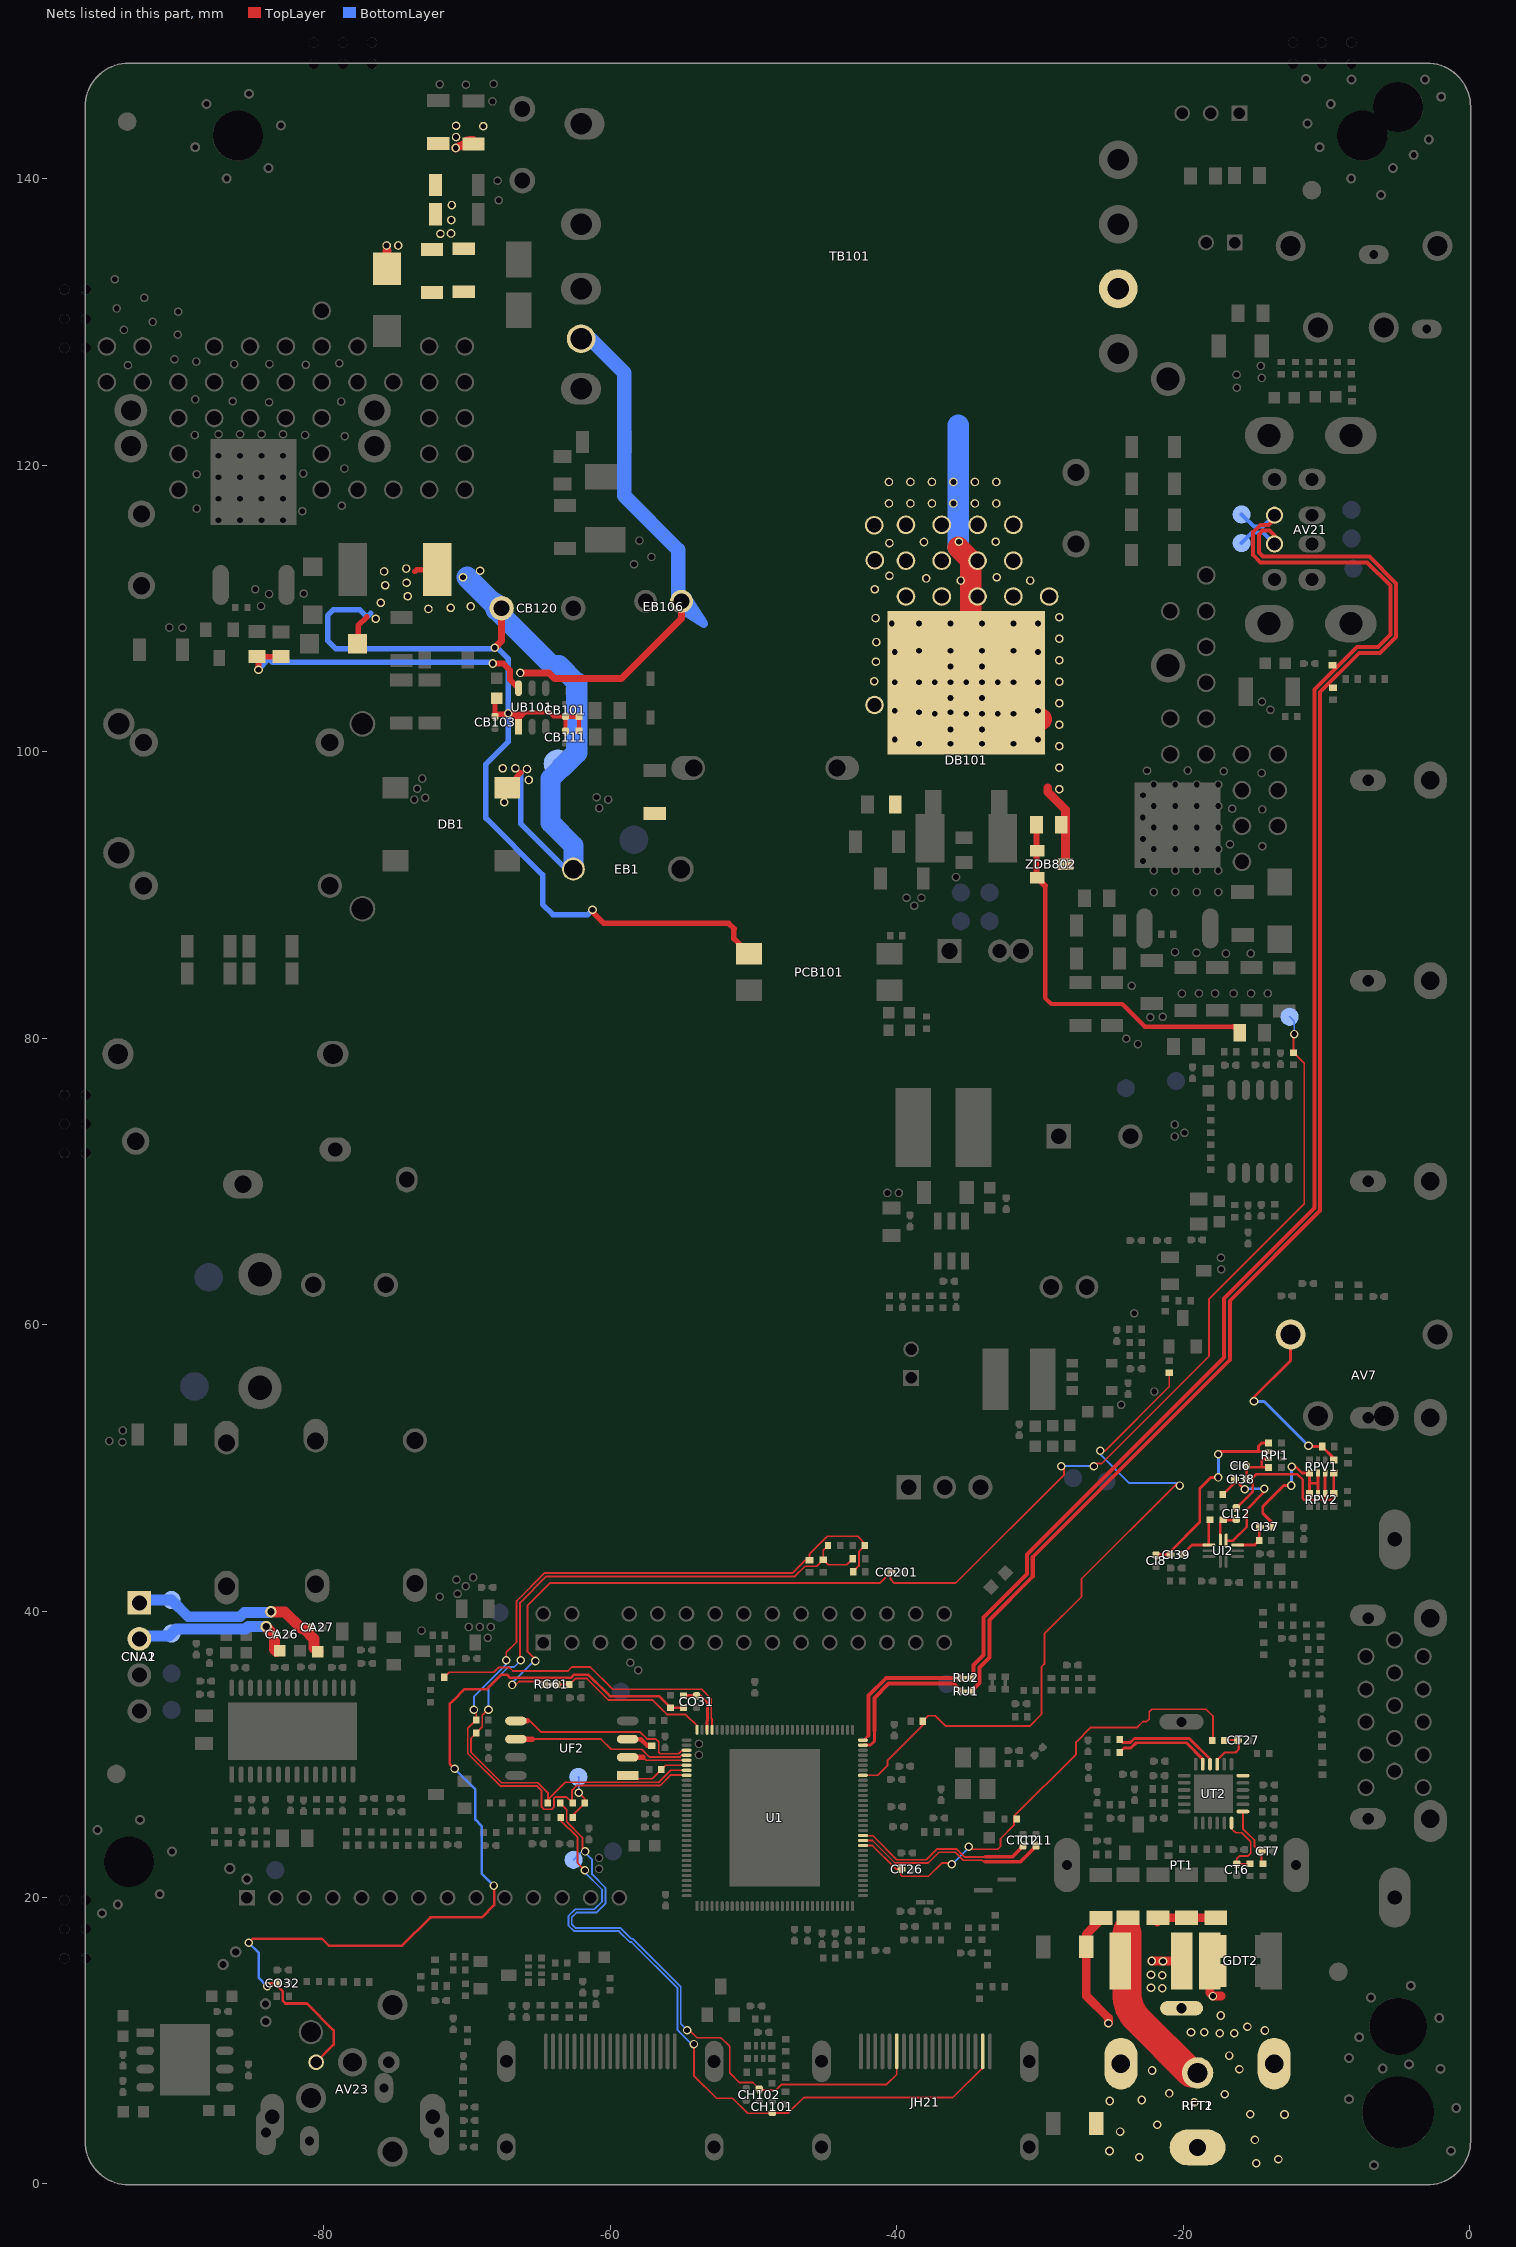
[diagram p0: the nets of this part, all layers, seen from the top]
# Altium PCB MISC86372.PcbDoc (part 13 of 16)
Units mm, origin at the board's own origin, x right, y up, seen from the top; angles counter-clockwise.
Board outline 96.73 x 148.13 mm, 2 copper layers (TopLayer, BottomLayer), stack 1.571 mm thick; 578 components, 318 nets, 2702 pads, 836 vias.

## Via types
v1: diameter 0.6, hole 0.4, TopLayer to BottomLayer, tented both sides, 816 vias
v2: diameter 0.7, hole 0.5, TopLayer to BottomLayer, tented both sides, 15 vias
v3: diameter 0.8, hole 0.5, TopLayer to BottomLayer, tented both sides, 5 vias

## Nets (pads, with @x,y where several pads share a name; then routed paths per layer and width w, separated by ;. In a path a pad name is that pad's centre, name@x,y a point inside that pad or via, vN(x,y) a via of type N, cw(c..) or ccw(c..) an arc to the next point about the centre after c; other vN are vias at no path point) (continued)
NetRB106_1: RB106.1 RB107.1 UB101.6 | length 23.3
  TopLayer w0.4: v1(-84.557,105.715) -84.557,106.627 -84.554,106.624 RB107.1@-82.982,106.624 ; -83.871,106.627 RB107.1@-82.906,106.627 ; v1(-68.199,106.147) -67.469,106.147 -66.996,105.674 -66.996,105.017 UB101.6@-66.406,104.427
  BottomLayer w0.4: v1(-84.557,105.715) -84.607,105.715 -83.829,106.493 -83.565,106.229 -68.281,106.229 v1(-68.199,106.147)
NetRB834_2: RB834.2 RB835.2 ZDB802.1 ZDB802.3 | length 26.9
  TopLayer w0.3: -29.642,90.627 -29.642,82.804 -29.211,82.373 -24.258,82.373 -22.682,80.797 RB834.2@-16.487,80.797
  TopLayer w0.4: RB835.2@-30.251,94.894 -30.251,91.237 ZDB802.3@-30.201,91.186 -29.642,90.627 ; RB834.2@-16.487,80.797 RB834.2@-16.055,80.366
NetRF23_1: RF23.1 UF2.3 | length 1.9
  TopLayer w0.305: UF2.3@-58.787,31.055 -57.869,31.055 -57.419,30.604 RF23.1@-57.099,30.604
NetRH102_2: RH102.2 RH105.1 RXD.1 | length 3.5
  TopLayer w0.127: RH102.2@-62.669,25.578 -62.669,25.705 RH105.1@-61.78,26.594 -61.78,26.88 v1(-62.205,27.305) v1@-62.255,27.254
  BottomLayer w0.127: RXD.1@-62.23,28.423 -62.205,28.397 v1(-62.205,27.305)
PANEL_EN_OUT_IC: RM11.1 U1.93 | length 22.3
  TopLayer w0.127: RM11.1@-71.603,35.377 -71.248,35.731 -68.136,35.731 -67.8,36.068 -67.048,36.068 -66.794,35.814 -62.956,35.814 -62.677,36.093 -61.392,36.093 -59.833,34.535 -56.159,34.535 -53.627,34.535 -52.952,33.86 -52.952,32.505 -52.885,32.438 -52.888,32.434 U1.93@-52.888,31.707 U1.93@-52.888,31.656
PC_L&AV_L: CI37.2@-13.85,45.868 CI37.2@-14.025,45.868 RPV1.6 RPV1.8 RPV2.2 RPV2.4 | length 10.4
  TopLayer w0.203: CI37.2@-13.85,45.868 -13.85,46.234 -14.448,46.832 -14.448,47.3 -12.983,48.765 v1(-12.453,48.765) ; v1(-12.421,50.063) -12.135,50.063 -11.703,49.632 RPV1.8@-11.192,49.632 -11.192,48.92 ; RPV2.2@-11.192,48.209 -11.192,48.692 -11.192,48.92 ; RPV2.4@-10.592,48.209 -10.592,48.946 ; RPV1.6@-10.592,49.632 -10.592,48.946 ; -11.192,48.92 -10.617,48.92 -10.592,48.946
  BottomLayer w0.203: v1(-12.453,48.765) v1@-12.453,50.031
PC_LIN_SW: CI37.1 RI37.1 UI2.10 | length 2.6
  TopLayer w0.178: UI2.10@-16.206,44.608 -15.02,44.608 RI37.1@-14.7,44.929 CI37.1@-14.7,45.868
PC_R: AV7.3 DV8.K RPV1.1 | length 13.7
  TopLayer w0.203: v1(-15.062,54.635) -15.062,54.933 -12.5,57.495 AV7.3@-12.5,59.3 AV7.3@-12.776,59.024 ; v1@-11.201,51.486 DV8.K@-10.306,51.486 -9.492,50.672 RPV1.1@-9.492,50.532
  BottomLayer w0.203: v1(-15.062,54.635) -14.351,54.635 v1@-11.328,51.613 ; AV7.3@-12.802,58.998 AV7.3@-12.5,59.3
  other v1: -11.252,51.537
PC_R&AV_R: CI12.2@-16.298,47.23 CI12.2@-16.298,47.055 RPV1.2 RPV1.4 RPV2.6 RPV2.8 | length 13.8
  TopLayer w0.178: CI12.2@-16.298,47.23 -16.245,47.23 -15.161,48.313 -15.161,49.276 -14.877,49.56 -12.044,49.56 -11.658,49.174 -11.658,47.87 -11.547,47.759 -10.178,47.759 ; RPV2.6@-10.092,48.209 -10.084,48.201 -10.084,47.854 -10.178,47.759 ; RPV1.4@-10.092,49.632 RPV1.4@-10.092,49.801 ; RPV2.8@-9.492,48.209 -9.492,47.836 -9.569,47.759 -10.178,47.759
  TopLayer w0.203: RPV2.6@-10.092,48.209 RPV1.4@-10.092,49.632 ; RPV2.8@-9.492,48.209 RPV1.2@-9.492,49.632
PC_RIN_SW: CI12.1 RI38.1 UI2.2 | length 2.3
  TopLayer w0.178: UI2.2@-17.406,44.958 -17.406,46.186 RI38.1@-17.213,46.38 ; -16.838,46.352 -16.836,46.354
  TopLayer w0.203: RI38.1@-17.085,46.354 -16.836,46.354 ; -16.838,46.352 -16.326,46.352 CI12.1@-16.298,46.38
POWER_EN_OUT_IC: RM1.1 RM2.1 U1.57 | length 49.4
  TopLayer w0.127: U1.57@-42.362,28.531 -41.327,28.531 -40.653,29.204 -40.653,29.541 RM1.1@-38.101,32.093 ; RM1.1@-38.183,32.309 -37.803,32.689 -37.309,32.689 -36.59,31.97 -30.728,31.97 -29.893,32.804 -29.893,36.108 -29.693,36.309 -29.693,38.405 -27.102,40.996 -27.102,42.24 v1@-20.418,48.924 ; v1(-25.794,51.194) -25.46,51.194 -20.98,55.673 RM2.1@-20.98,56.623
  BottomLayer w0.127: v1(-25.794,51.194) -25.794,50.947 -23.78,48.933 -20.426,48.933 v1(-20.25,48.757)
PWM1: RF13.1 RG61.1 U1.96 | length 11.6
  TopLayer w0.127: RG61.1@-63.71,34.87 RF13.1@-62.858,34.87 -62.443,35.285 -61.625,35.285 -60.122,33.782 -57.039,33.782 -56.413,33.157 -56.032,32.775 -55.711,32.775 -55.702,32.766 -54.725,32.766 -53.938,31.979 U1.96@-53.938,31.707 U1.96@-53.938,31.656
PWM_REF: CG201.1 PWM_REF.1 RB813.1 RG61.2 RG61.3 | length 92.7
  TopLayer w0.127: v1@-66.754,34.693 -66.37,35.077 -64.767,35.077 RG61.2@-64.56,34.87 ; -65.786,37.795 -65.786,38.278 ; v1(-65.227,36.508) -65.227,36.627 -65.786,37.186 -65.786,38.278 ; v1@-28.321,49.911 -28.321,49.527 -35.897,41.951 -40.173,41.951 -40.43,42.208 CG201.1@-40.43,42.723 -41.201,41.951 -64.215,41.951 -65.786,40.38 -65.786,38.278 ; v1@-26.054,50.298 -25.698,50.298 -18.194,57.802 -18.194,61.79 -11.557,68.427 -11.557,78.251 RB813.1@-12.294,78.987 -12.294,80.233 v1(-12.248,80.278) v1@-12.248,80.309
  BottomLayer w0.127: v1(-66.837,34.841) -66.837,34.992 -66.345,35.484 ; v1@-66.754,35.075 -66.345,35.484 ; v1@-65.275,36.555 -66.345,35.484 ; v1(-28.524,50.114) v1(-26.238,50.114) ; PWM_REF.1@-12.573,81.483 -12.248,81.159 v1(-12.248,80.278)
RF_INPUT: CT13.1 GDT1.1 RFT1.1 RFT2.1 | length 12.2
  TopLayer w1.905: GDT1.1@-23.933,17.522 -23.933,17.767
  TopLayer w2.032: GDT1.1@-23.925,17.514 -23.925,13.267 ccw(c-21.385,13.267) -23.181,11.471 -19.461,7.75 RFT1.1@-19,7.75
RFGND: CT41.2 CT42.2 CT43.2 CT44.2 CT45.2 CT46.2 CT47.2 CT48.2 GDT1.2 GDT2.1@-17.501,14.554 GDT2.1@-17.502,16.586 GDT2.1@-18.152,15.57 PT1.1 RFT1.2 RFT1.3 RFT1.4 RFT2.2 RFT2.3 RFT2.4 | length 18
  TopLayer w0.61: CT41.2@-25.754,18.566 -25.754,18.446 -26.77,17.43 CT47.2@-26.77,16.561 -26.77,13.13 -25.222,11.582 v1(-25.222,11.227) ; v1(-22.2,15.57) GDT1.2@-20.1,15.57 ; CT42.2@-21.817,18.289 -21.817,18.591 CT44.2@-17.753,18.591 ; GDT2.1@-18.152,15.57 -18.152,13.343 v1(-17.927,13.118) -17.342,13.118
  other v1: -14.901,1.448 -13.356,1.727 -23.067,1.86 -25.146,2.3 -14.994,3.076 -24.409,3.658 -21.819,4.14 -12.929,4.851 -15.316,4.877 -19.228,5.69 -25.132,5.791 -22.9,5.865 -17.094,6.274 -20.98,6.325 -22.173,7.924 -16.078,8.001 -16.789,8.966 -17.45,10.516 -16.434,10.516 -19.456,10.59 -18.542,10.592 -14.3,10.718 -15.519,10.973 -17.374,11.76 -21.463,13.665 -22.25,13.691 -21.463,14.58 -22.25,14.605 -21.412,15.545
ROUT+: BA4.2 CA27.1 CNA1.1 CNA2.1 pad.VIA5@-83.693,39.954 ROUT+.1 | length 14.6
  TopLayer w0.762: pad.VIA5@-83.693,39.929 -82.724,39.929 -81.563,38.767 -81.4,38.767 -80.683,38.051 -80.683,37.432 BA4.2@-80.412,37.16
  BottomLayer w0.762: CNA1.1@-92.877,40.773 -90.634,40.773 ROUT+.1@-90.627,40.767 -89.462,39.601 -85.855,39.601 -85.553,39.903 pad.VIA5@-83.693,39.903
ROUT-: BA3.2 CA26.2@-83.177,38.372 CA26.2@-83.352,38.372 CNA1.2 CNA2.2 pad.VIA5@-84.023,38.913 ROUT-.1 | length 10.9
  TopLayer w0.254: -83.687,37.668 -83.687,38.179
  TopLayer w0.762: pad.VIA5@-84.023,38.913 -84.023,38.875 -83.687,38.538 ; -83.433,37.922 -83.433,37.322 BA3.2@-83.298,37.188
  BottomLayer w0.762: CNA1.2@-92.877,38.253 -90.804,38.253 ROUT-.1@-90.627,38.43 -90.32,38.738 -85.468,38.738 -85.293,38.913 pad.VIA5@-84.023,38.913
RXD: CH101.2@-48.692,4.96 CH101.2@-48.692,5.135 JH21.2 RH102.1 | length 50
  TopLayer w0.127: RH102.1@-63.519,25.578 -63.519,25.441 -62.281,24.204 -62.281,22.403 v1(-61.773,21.895) ; v1(-54.161,9.765) -54.161,7.57 -52.583,5.991 -51.465,5.991 -50.413,4.938 -49.298,4.938 ; -49.294,4.942 -48.819,4.942 -48.819,4.96 -47.566,4.96 -46.488,6.037 -36.09,6.037 -34,8.127 JH21.2@-34,9.258
  BottomLayer w0.127: v1@-61.773,21.753 -60.579,20.559 -60.579,19.714 -61.116,19.177 -62.452,19.177 -62.916,18.713 -62.916,18.041 -62.528,17.653 -59.398,17.653 -58.636,16.891 -58.522,16.891 -55.304,13.673 -55.304,10.743 v1@-54.326,9.765
SC_AU_LIN_C: CI6.2@-15.582,50.126 CI6.2@-15.757,50.126 CI38.2@-15.577,49.2 CI38.2@-15.752,49.2 RPI1.2 RPI1.4 | length 3.5
  TopLayer w0.178: -15.582,49.842 CI6.2@-15.582,50.126 ; CI38.2@-15.577,49.2 -15.582,49.205 CI6.2@-15.582,50.126 ; -14.503,50.063 -14.503,50.521 -14.398,50.626 -14.308,50.626 ; RPI1.2@-14.039,50.026 -15.482,50.026 CI6.2@-15.582,50.126
SC_AU_LIN_SW: CI38.1 RI39.1 UI2.1 | length 8.9
  TopLayer w0.178: RI39.1@-17.228,48.148 RI39.1@-17.228,48.133 -16.427,48.934 ; UI2.1@-17.006,44.908 -16.526,44.908 -15.553,45.882 -15.553,47.096 -14.351,48.297 v1(-14.351,48.539) ; -16.427,48.913 CI38.1@-16.427,49.2 -15.724,48.497 v1(-15.711,48.497) ; CI38.1@-16.252,49.124 CI38.1@-16.252,49.2
  BottomLayer w0.178: v1(-15.711,48.497) -15.669,48.539 v1(-14.351,48.539)
SC_AU_RIN_C: CI8.2@-21.895,43.76 CI8.2@-21.895,43.935 CI39.2@-20.752,43.94 CI39.2@-20.927,43.94 RPI1.6 RPI1.8 | length 14.3
  TopLayer w0.203: CI8.2@-21.895,43.935 CI39.2@-20.931,43.935 ; CI39.2@-20.927,44.124 -18.847,46.204 -18.847,48.561 -18.081,49.327 v1(-17.552,49.327) ; v1(-17.552,50.952) -17.378,51.126 -16.951,51.126 ; -16.971,51.126 -16.951,51.126 ; RPI1.6@-14.039,51.126 -14.732,51.126 ; RPI1.8@-14.039,51.726 -14.523,51.726 -14.732,51.517 -14.732,51.126 ; -16.951,51.126 -14.732,51.126
  BottomLayer w0.203: v1@-17.544,49.327 v1@-17.544,50.952
SC_AU_RIN_SW: CI39.1 RI40.1 UI2.3 | length 4
  TopLayer w0.178: -19.379,44.608 UI2.3@-18.206,44.608 -18.206,46.301 RI40.1@-18.127,46.38
  TopLayer w0.203: CI39.1@-20.098,43.889 -19.379,44.608
SGND: CB101.2@-63.129,102.62 CB101.2@-63.129,102.445 CB102.2 CB103.2@-68.047,102.282 CB103.2@-68.047,102.457 CB111.1 CB120.1 DB1.4 DB110.K EB1.2@-62.576,91.796 EB106.2 pad.VIA5@-65.684,98.019 pad.VIA5@-65.811,98.781 pad.VIA5@-66.624,98.831 pad.VIA5@-67.412,96.469 pad.VIA5@-67.513,98.831 pad.VIA5@-69.088,112.624 pad.VIA5@-69.748,110.134 pad.VIA5@-70.282,112.166 pad.VIA5@-71.145,110.033 pad.VIA5@-72.695,109.957 pad.VIA5@-74.143,110.846 pad.VIA5@-74.219,111.785 pad.VIA5@-74.244,112.776 pad.VIA5@-75.717,111.608 pad.VIA5@-75.794,112.573 pad.VIA5@-76.022,110.388 pad.VIA5@-76.378,109.271 PCB101.3 RB103.1 RB104.1 RB130.1 RB148.1 TB101.5 TP-TDT.2 UB101.1 | length 143.7
  TopLayer w0.3: UB101.1@-66.406,102.245 -65.927,102.724 -64.237,102.724 -63.957,102.445 CB101.2@-63.129,102.445 ; -63.129,101.847 CB111.1@-63.129,101.441 CB101.2@-63.129,102.445 ; RB104.1@-62.189,101.441 RB103.1@-62.189,102.42 -63.103,102.42 CB101.2@-63.129,102.445
  TopLayer w0.381: DB110.K@-77.597,107.366 -77.597,108.788 -76.987,109.398 ; -73.635,112.573 -73.508,112.7 RB148.1@-72.082,112.7 ; CB103.2@-68.047,102.562 CB102.2@-68.047,103.815 ; CB103.2@-68.021,102.591 -66.751,102.591 ; DB1.4@-66.878,97.892 -66.243,98.527 ; UB101.1@-66.406,102.245 -66.751,102.591 ; -66.142,102.591 -66.751,102.591 ; v1(-61.239,88.951) -61.239,88.794 -60.452,88.007 -51.731,88.007 -51.358,87.634 -51.365,87.627 -51.365,86.944 -49.957,85.536 PCB101.3@-49.957,85.522
  TopLayer w0.5: v1(-68.072,107.239) -67.586,107.725 CB120.1@-67.586,110.007 ; v1(-66.29,105.49) -64.274,105.49 -63.89,105.105 -59.207,105.105 -55.031,109.282 EB106.2@-55.031,110.49
  BottomLayer w0.381: -76.721,109.664 -76.987,109.398 -77.495,109.906 -79.324,109.906 -79.731,109.499 -79.731,107.74 -79.177,107.186 v1@-68.072,107.186 ; v1@-67.835,107.186 -67.132,106.483 v1(-67.132,102.667) -67.132,100.677 -68.682,99.128 -68.682,95.352 -64.719,91.389 -64.719,89.332 -64.008,88.621 -61.57,88.621 v1(-61.239,88.951) ; -66.243,98.527 -66.243,94.945 -63.094,91.796 EB1.2@-62.576,91.796
  BottomLayer w1: TB101.5@-62.038,128.819 -61.408,128.819 -59.03,126.441 -59.03,117.856 -55.265,114.091 EB106.2@-55.265,110.236
  BottomLayer w1.4: CB120.1@-67.829,109.764 -64.096,106.032 -63.573,106.032 -62.357,104.816 ; TP-TDT.2@-63.076,99.205 -64.16,98.12 -64.16,95.021 -62.576,93.437 EB1.2@-62.576,91.796
  BottomLayer w1.5: pad.VIA5@-69.999,112.166 CB120.1@-67.958,110.126 ; CB120.1@-67.958,109.894 CB120.1@-67.958,110.126 ; CB120.1@-67.586,109.753 CB120.1@-67.958,110.126 ; TP-TDT.2@-63.39,98.89 -62.357,99.924 -62.357,104.816
SNB-D: DB106.K pad.VIA5@-68.859,143.662 pad.VIA5@-70.79,142.138 pad.VIA5@-70.764,142.9 pad.VIA5@-70.764,143.688 pad.VIA5@-74.803,135.331 pad.VIA5@-75.616,135.331 RB117.1 RB118.1 RB150.1 RB151.1 | length 3.3
  TopLayer w0.6: DB106.K@-75.59,133.706 -75.59,134.976 ; pad.VIA5@-70.79,142.138 RB117.1@-69.897,142.54 ; RB117.1@-69.774,142.416 RB117.1@-69.897,142.54 ; RB117.1@-69.897,142.54 -69.672,142.641 -69.629,142.66 -69.586,142.68 -69.799,142.667 -70.004,142.646 RB117.1@-69.897,142.54
SNB-RM: pad.VIA5@-71.12,136.169 pad.VIA5@-71.065,138.151 pad.VIA5@-71.095,137.109 pad.VIA5@-71.857,136.144 RB150.2 RB151.2 RB152.1 RB153.1
SPDIF_OUT: AV23.1 CO32.2@-83.28,14.021 CO32.2@-83.105,14.021 RO21.2 RO22.2 | length 65.4
  TopLayer w0.178: v1(-85.242,16.84) -84.963,17.12 -80.137,17.12 -79.654,16.637 -74.534,16.637 -72.553,18.618 -68.971,18.618 -68.116,19.473 v1@-68.116,20.805 ; v1(-83.952,13.797) -83.728,14.021 CO32.2@-83.28,14.021 ; CO32.2@-83.28,13.851 -82.855,13.426 -82.855,12.776 -82.677,12.598 -81.178,12.598 -79.308,10.728 -79.308,9.732 AV23.1@-80.54,8.5 ; v1(-70.872,28.989) -71.144,29.262 -71.222,29.339 -71.222,33.506 -70.995,33.733 -70.184,34.544 -68.605,34.544 -67.589,35.56 -67.222,35.56 -66.993,35.331 -62.756,35.331 -62.528,35.56 -61.541,35.56 -61.026,35.046 ; -61.287,35.306 -60.033,34.052 -56.6,34.052 RO22.2@-55.804,33.255 RO22.2@-55.702,33.255 ; RO22.2@-55.753,33.306 RO22.2@-55.702,33.255 ; RO22.2@-55.695,33.249 RO22.2@-55.702,33.255 ; RO21.2@-54.88,33.249 -54.886,33.255 RO22.2@-55.702,33.255
  BottomLayer w0.178: v1(-85.242,16.84) -84.557,16.154 -84.557,14.401 v1(-83.952,13.797) ; v1(-70.872,28.989) -69.425,27.542 -69.425,25.432 -68.982,24.989 -68.982,21.671 v1(-68.144,20.833)
SPDIF_OUT_IC: CO31.2@-53.975,33.931 CO31.2@-53.975,34.106 RO21.1 U1.94 | length 3.8
  TopLayer w0.203: RO21.1@-54.845,34.163 -54.788,34.106 CO31.2@-53.975,34.106 ; CO31.2@-53.95,34.106 CO31.2@-53.975,34.106 ; U1.94@-53.238,31.656 U1.94@-53.238,31.707 -53.238,32.334 -53.219,32.354 -53.219,33.615 -53.709,34.106 CO31.2@-53.975,34.106
SPI_CLK: U1.100 UF2.6 | length 12.6
  TopLayer w0.127: -65.441,31.055 -60.646,31.055 -59.944,30.353 -57.809,30.353 -57.265,29.809 -55.138,29.809 -55.016,29.931 U1.100@-54.663,29.931
  TopLayer w0.381: UF2.6@-66.707,31.055 -65.441,31.055
SPI_CSN: RF3.1 U1.102 UF2.1 | length 4.6
  TopLayer w0.127: UF2.1@-58.787,28.515 -58.559,28.286 -57.085,28.286 RF3.1@-56.44,28.931 -56.14,29.231 U1.102@-54.664,29.231
SPI_DI: U1.99 UF2.5 | length 13.4
  TopLayer w0.127: -65.799,32.325 -65.619,32.325 -64.857,31.563 -57.928,31.563 -57.429,31.064 -56.82,31.064 -56.617,30.861 -56.617,30.15 -56.505,30.038 -55.232,30.038 -54.99,30.281 U1.99@-54.613,30.281
  TopLayer w0.381: UF2.5@-66.587,32.325 -65.799,32.325
SPI_DO: U1.101 UF2.2 | length 4.2
  TopLayer w0.127: -57.744,29.785 -57.699,29.785 -57.495,29.581 U1.101@-54.664,29.581
  TopLayer w0.381: UF2.2@-58.787,29.785 -57.744,29.785
SYN: CB117.1 DB101.2 pad.VIA5@-28.651,97.378 pad.VIA5@-28.651,98.878 pad.VIA5@-28.651,100.378 pad.VIA5@-28.651,101.878 pad.VIA5@-28.651,103.378 pad.VIA5@-28.651,104.878 pad.VIA5@-28.651,106.378 pad.VIA5@-28.651,107.878 pad.VIA5@-28.651,109.378 pad.VIA5@-29.359,110.827 pad.VIA5@-30.683,111.938 pad.VIA5@-31.859,110.827 pad.VIA5@-31.859,113.327 pad.VIA5@-31.859,115.827 pad.VIA5@-33.02,112.166 pad.VIA5@-33.045,117.321 pad.VIA5@-33.045,118.821 pad.VIA5@-33.096,114.656 pad.VIA5@-34.359,110.827 pad.VIA5@-34.359,113.327 pad.VIA5@-34.359,115.827 pad.VIA5@-34.545,117.321 pad.VIA5@-34.545,118.821 pad.VIA5@-35.535,111.938 pad.VIA5@-35.662,114.656 pad.VIA5@-36.045,117.321 pad.VIA5@-36.045,118.821 pad.VIA5@-36.859,110.827 pad.VIA5@-36.859,113.327 pad.VIA5@-36.859,115.827 pad.VIA5@-37.545,117.321 pad.VIA5@-37.545,118.821 pad.VIA5@-37.948,112.09 pad.VIA5@-38.1,114.63 pad.VIA5@-39.045,117.321 pad.VIA5@-39.045,118.821 pad.VIA5@-39.359,110.827 pad.VIA5@-39.359,113.327 pad.VIA5@-39.359,115.827 pad.VIA5@-40.513,112.268 pad.VIA5@-40.513,114.554 pad.VIA5@-40.545,117.321 pad.VIA5@-40.545,118.821 pad.VIA5@-41.58,104.902 pad.VIA5@-41.58,115.799 pad.VIA5@-41.427,107.645 pad.VIA5@-41.453,106.274 pad.VIA5@-41.478,109.322 pad.VIA5@-41.529,111.328 pad.VIA5@-41.529,113.36 pad.VIA5@-41.554,103.251 RB835.1 TB101.8 ZDB802.2 | length 29.8
  TopLayer w0.6: -29.464,97.485 -29.464,97.18 -28.219,95.935 ZDB802.2@-28.219,92.138
  TopLayer w1.5: -35.712,114.249 -34.849,113.386 -34.849,110.827 -34.849,107.046 -34.849,105.513 -34.643,105.307 -33.562,104.226 -31.596,102.26 DB101.2@-29.896,102.26
  BottomLayer w1.5: -35.712,114.249 -35.712,117.321 -35.712,122.784
  other v1: -38.442,100.546 -36.242,100.546 -34.042,100.546 -31.842,100.546 -40.142,100.846 -30.142,100.846 -36.242,101.546 -34.042,101.546 -37.342,102.646 -35.142,102.646 -34.042,102.646 -32.942,102.646 -31.842,102.646 -38.442,102.746 -36.242,102.746 -40.142,102.846 -30.142,102.846 -36.242,103.746 -34.042,103.746 -40.142,104.846 -38.442,104.846 -37.342,104.846 -36.242,104.846 -35.142,104.846 -34.042,104.846 -32.942,104.846 -31.842,104.846 -30.142,104.846 -36.242,105.946 -34.042,105.946 -40.142,106.946 -30.142,106.946 -38.442,107.046 -36.242,107.046 -34.042,107.046 -31.842,107.046 -40.342,108.946 -38.442,108.946 -36.242,108.946 -34.042,108.946 -31.842,108.946 -30.142,108.946
TUNER_AGC_OUT: CT27.2@-16.049,30.963 CT27.2@-16.224,30.963 RT8.1 UT2.15 | length 3.5
  TopLayer w0.152: UT2.15@-17.632,29.304 -17.632,29.595 -17.103,30.124 -16.358,30.124 -16.122,30.36 CT27.2@-16.122,30.836 ; RT8.1@-17.025,30.988 CT27.2@-16.122,30.988
TUNER_AGC_OUT_IC: CT26.2@-39.544,21.971 CT26.2@-39.719,21.971 RT7.2 RT8.2 U1.43 | length 35.6
  TopLayer w0.127: U1.43@-42.363,23.631 -41.701,23.631 -40.042,21.971 CT26.2@-39.719,21.971 ; CT26.2@-39.694,21.971 CT26.2@-39.719,21.971 ; v1@-36.424,22.403 -36.859,22.403 ; v1(-36.17,22.327) -36.246,22.403 -36.859,22.403 ; v1(-34.976,23.546) -34.798,23.368 -33.934,23.368 ; v1@-34.874,23.368 -33.934,23.368 ; RT8.2@-17.932,30.963 -17.932,32.67 -18.41,33.147 -22.199,33.147 -22.371,32.975 -22.371,32.455 -22.542,32.285 -22.812,32.285 -23.22,31.877 -26.455,31.877 -27.485,30.847 -27.485,30.008 -31.823,25.669 -31.823,25.039 -32.756,24.107 -32.756,23.563 -32.951,23.368 -33.934,23.368 ; CT26.2@-39.719,21.971 -39.719,21.596 -39.602,21.48 -37.782,21.48 -36.859,22.403
  BottomLayer w0.127: v1@-36.424,22.403 -36.043,22.403 v1@-34.976,23.47
TUNER_IF_N_IN: RT5.1 UT2.16 | length 7.5
  TopLayer w0.203: RT5.1@-24.442,31.039 -24.213,30.81 -23.709,30.81 -23.411,31.109 -19.577,31.109 -18.132,29.663 UT2.16@-18.132,29.304
TUNER_IF_N_IN_IC: CT12.1 U1.45 | length 12.7
  TopLayer w0.127: U1.45@-42.338,24.306 -41.658,24.306 -39.991,22.638 -37.938,22.638 -37.182,23.393 -35.832,23.393 -35.274,22.835 -33.878,22.835 -33.865,22.847 -33.815,22.847
  TopLayer w0.254: -33.815,22.847 -31.922,22.847 CT12.1@-31.191,23.578
TUNER_IF_P_IN: RT4.1 UT2.17 | length 6.9
  TopLayer w0.203: RT4.1@-24.442,30.124 -24.137,30.429 -23.659,30.429 -23.285,30.804 -19.78,30.804 -18.632,29.655 UT2.17@-18.632,29.304
TUNER_IF_P_IN_IC: CT11.1 U1.44 | length 13.8
  TopLayer w0.127: U1.44@-42.362,23.981 -41.692,23.981 -40.121,22.41 -37.807,22.41 -37.052,23.165 -35.927,23.165 -35.368,22.606 -34.04,22.606 -33.925,22.492 -33.807,22.492
  TopLayer w0.254: -33.807,22.492 -31.363,22.492 CT11.1@-30.277,23.578
TUNER_SCL_OUT: CT6.2@-16.259,22.2 CT6.2@-16.259,22.375 RT2.2 UT2.6 | length 5.3
  TopLayer w0.127: UT2.6@-16.632,25.204 -16.632,24.81 -16.34,24.519 -15.9,24.519 -15.288,23.907 -15.288,23.08 -15.466,22.902 -16.061,22.902 -16.259,22.704 -16.259,22.349 -15.37,22.349 RT2.2@-15.345,22.324
TUNER_SDA_IO: CT7.2@-14.367,23.239 CT7.2@-14.542,23.239 RT3.2 UT2.7 | length 4.6
  TopLayer w0.127: UT2.7@-15.832,26.004 -15.832,24.809 -15.034,24.012 -15.034,23.571 -14.703,23.239 CT7.2@-14.542,23.239 ; CT7.2@-14.542,23.341 CT7.2@-14.542,23.239 ; CT7.2@-14.542,23.418 CT7.2@-14.542,23.239 ; RT3.2@-14.43,22.324 -14.542,22.435 CT7.2@-14.542,23.239
TUNER_XTAL_IN: UT2.12
TXD: CH102.2@-49.604,6.473 CH102.2@-49.604,6.648 JH21.14 RH103.1 TXD.1 | length 44.9
  TopLayer w0.127: RH103.1@-63.507,26.594 -63.043,26.13 -63.043,25.289 -61.943,24.189 -61.943,23.403 v1(-61.758,23.219) ; v1(-54.638,10.735) -54.474,10.735 -53.945,10.206 -52.269,10.206 -51.664,9.601 -51.664,7.752 -50.995,7.083 -50.038,7.083 CH102.2@-49.604,6.648 CH102.2@-49.526,6.57 ; CH102.2@-49.663,6.57 CH102.2@-49.526,6.57 ; CH102.2@-49.522,6.566 CH102.2@-49.526,6.57 ; JH21.14@-40,9.258 -40,7.643 -40.693,6.95 -48.028,6.95 -48.408,6.57 CH102.2@-49.526,6.57
  BottomLayer w0.127: TXD.1@-62.56,22.631 -61.973,23.219 v1(-61.758,23.219) -61.758,23.125 -61.273,22.639 -61.273,21.612 -60.325,20.664 -60.325,19.609 -60.985,18.948 -62.357,18.948 -62.687,18.618 -62.687,18.136 -62.433,17.882 -59.304,17.882 -58.542,17.12 -58.427,17.12 -55.075,13.768 -55.075,11.172 v1(-54.638,10.735)
UART_RX_IC: CD101.K RF8.1 RF11.1 RH105.2 RH106.1 U1.104 | length 61.4
  TopLayer w0.127: -69.954,30.41 -69.954,30.683 ; v1@-69.361,32.953 RH106.1@-69.361,32.401 -69.954,31.808 -69.954,30.683 ; -67.331,27.788 -67.132,27.788 ; v1(-67.264,36.558) -67.264,37.117 -66.548,37.833 -66.548,40.696 -64.598,42.646 -47.981,42.646 -47.286,42.646 -46.387,43.545 CD101.K@-46.096,43.545 -46.096,43.975 -45.163,44.908 ; RH105.2@-62.63,26.594 RH105.2@-62.67,26.634 ; -58.699,27.821 -58.623,27.821 ; U1.104@-54.664,28.531 -55.041,28.531 -55.068,28.557 -55.771,28.557 -56.507,27.821 -58.623,27.821 ; -45.008,45.063 -45.163,44.908 ; RF11.1@-43.046,42.739 -42.639,43.146 -42.639,44.147 RF8.1@-42.222,44.564 ; RF8.1@-42.222,44.716 -42.721,45.215 -44.856,45.215 -45.163,44.908 ; -69.954,30.683 -69.954,30.055 -67.687,27.788 -67.132,27.788 ; -67.132,27.788 -65.144,27.788 -64.795,27.439 -64.795,26.324 -64.633,26.162 -64.08,26.162 -63.932,26.31 -63.932,26.924 -63.847,27.009 -63.045,27.009 RH105.2@-62.67,26.634 ; RH105.2@-62.67,26.634 -62.67,27.501 -62.349,27.821 -59.064,27.821 -58.623,27.821
  BottomLayer w0.127: v1(-69.52,33.112) v1@-69.52,33.374 ; v1@-69.52,33.366 -69.52,34.025 -67.264,36.281 v1(-67.264,36.558)
UART_TX_IC: CD102.K RF9.1 RF10.1 RH103.2 RH104.1 U1.103 | length 56.4
  TopLayer w0.127: -69.725,30.251 -69.725,30.556 ; v1(-68.504,33.112) -68.544,33.112 -68.936,32.72 -68.936,31.912 RH104.1@-69.361,31.487 -69.725,31.122 -69.725,30.556 ; -66.294,37.42 -66.294,37.643 ; -66.294,37.846 -66.294,38.1 ; v1(-66.252,36.558) -66.294,36.6 -66.294,37.643 ; RH103.2@-64.357,26.594 -64.357,27.324 -65.049,28.016 -67.592,28.016 -69.725,30.149 -69.725,30.556 ; RH103.2@-64.357,26.822 -63.13,28.049 -56.602,28.049 -55.771,28.881 U1.103@-54.664,28.881 ; RF9.1@-44.799,44.564 -45.131,44.232 CD102.K@-45.131,43.57 ; RF10.1@-43.064,43.649 -43.489,43.224 -44.785,43.224 CD102.K@-45.131,43.57 ; -66.294,37.643 -66.294,38.1 ; -66.294,38.1 -66.294,40.591 -64.467,42.417 -47.108,42.417 -46.406,43.12 -45.581,43.12 CD102.K@-45.131,43.57
  BottomLayer w0.127: v1@-68.504,33.366 -68.504,34.717 -67.128,36.093 -66.717,36.093 v1(-66.252,36.558)
USB0_DM_IO: AV21.2 DM0.1 DU3.K RU1.2 RU1.3 | length 107
  TopLayer w0.279: RU1.2@-34.724,34.413 -34.724,34.475 -34.232,34.967 -34.232,36.062 -33.528,36.766 -33.528,39.385 -30.506,42.407 -30.506,43.767 -16.753,57.52 -16.753,61.65 -10.439,67.964 -10.439,104.156 -7.712,106.883 -6.248,106.883 -5.131,108.001 -5.131,111.747 -6.998,113.614 -14.427,113.614 -14.707,113.894 -14.707,115.164 -14.453,115.418 -13.97,115.418 -13.63,115.078 AV21.2@-13.63,114.5
  BottomLayer w0.279: DM0.1@-15.925,114.556 -15.19,115.291 -14.421,115.291 AV21.2@-13.63,114.5
USB0_DM_IO_IC: RU1.1 U1.63 | length 10.5
  TopLayer w0.203: U1.63@-42.352,30.642 -41.833,30.642 -41.561,30.914 -41.561,31.648
  TopLayer w0.279: -41.561,31.648 -41.561,33.929 -40.565,34.924 -36.023,34.924 -35.625,34.527 RU1.1@-35.625,34.413
USB0_DP_IO: AV21.3 DP0.1 DU4.K RU2.2 RU2.3 | length 106.4
  TopLayer w0.279: RU2.2@-34.724,35.327 -34.638,35.413 -34.638,36.231 -33.934,36.935 -33.934,39.554 -30.913,42.575 -30.913,43.936 -30.744,44.104 -17.479,57.369 -17.159,57.689 -17.159,61.818 -10.846,68.132 -10.846,104.324 -7.88,107.29 -6.417,107.29 -5.537,108.169 -5.537,111.579 -7.166,113.208 -14.596,113.208 -15.113,113.725 -15.113,115.332 -14.621,115.824 -14.046,115.824 -13.63,116.24 AV21.3@-13.63,116.5
  BottomLayer w0.279: DP0.1@-15.925,116.556 -15.066,115.697 -14.433,115.697 AV21.3@-13.63,116.5
USB0_DP_IO_IC: RU2.1 U1.64 | length 10
  TopLayer w0.178: U1.64@-42.362,30.981 -42.286,30.981 -41.968,31.3
  TopLayer w0.279: -41.968,31.3 -41.968,34.097 -40.734,35.331 RU2.1@-35.763,35.331